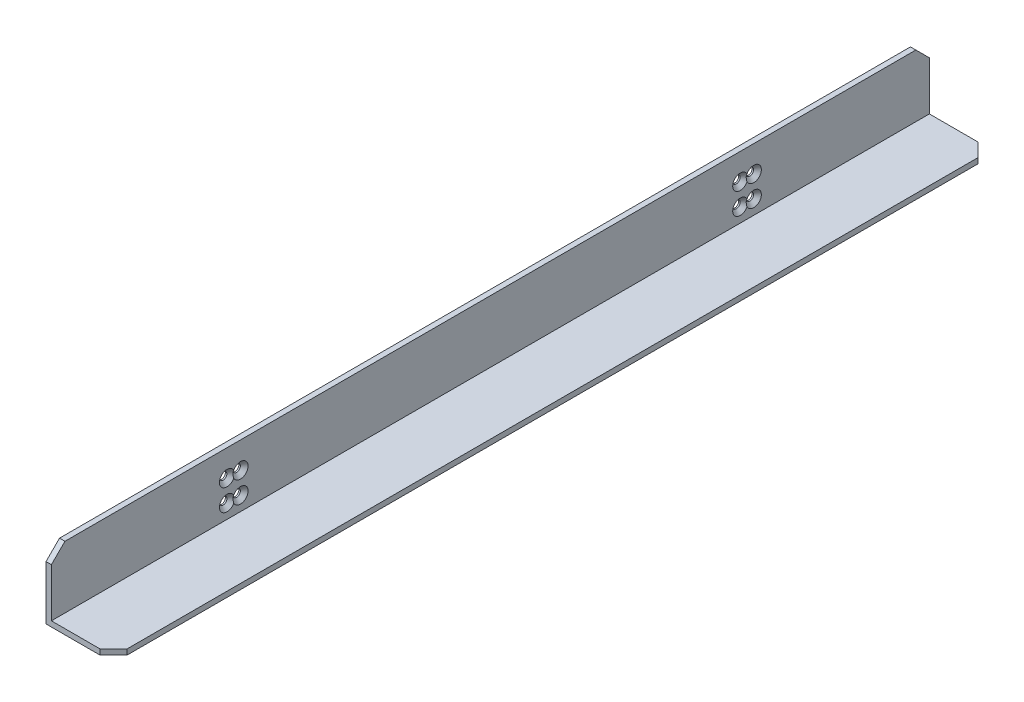
SolidWorks part; units mm, degrees
material "Q235A"
ref_plane "前视基准面" through (0, 0, 0) normal (0, 0, 1) x (1, 0, 0)
ref_plane "上视基准面" through (0, 0, 0) normal (0, 1, 0) x (1, 0, 0)
ref_plane "右视基准面" through (0, 0, 0) normal (1, 0, 0) x (0, 0, -1)
sketch "草图1" plane through (0, 0, 0) normal (0, 0, 1) x (1, 0, 0)
  line L0 (0, 0) -> (50, 0)
  line L1 (50, 0) -> (50, 4)
  line L2 (50, 4) -> (4, 4)
  line L3 (4, 4) -> (4, 50)
  line L4 (4, 50) -> (0, 50)
  line L5 (0, 50) -> (0, 0)
  dimension "D1" = 50
  dimension "D2" = 4
extrude "凸台-拉伸1" add sketch "草图1" along normal mid plane 650
chamfer "倒角1" distance 10 angle 45 4 edges at (50, 2, -325) (2, 50, -325) (50, 2, 325) (2, 50, 325)
hole_wizard "M5 六角凹锥坑螺钉的锥形沉头孔2" positions "草图4" profile "草图5" countersink size "M5" standard "ISO" end condition through all
sketch "草图4" plane through (4, 0, 0) normal (1, 0, 0) x (0, 0, -1)
  line L0 (185, 30.5) -> (195, 30.5) construction
  line L1 (185, 14.5) -> (195, 14.5) construction
  line L2 (195, 30.5) -> (195, 14.5) construction
  point P0 (-195, 30.5)
  point P3 (185, 30.5)
  point P9 (-185, 30.5)
  point P10 (195, 30.5)
  point P16 (-195, 14.5)
  point P17 (185, 14.5)
  point P18 (-185, 14.5)
  point P19 (195, 14.5)
  dimension "D2" = 10
  dimension "D4" = 16
  dimension "D1" = 2
  dimension "D3" = 2
sketch "草图5" plane through (4, 30.5, 195) normal (0, 1, 0) x (0, 0, -1)
  line L0 (0, 0) -> (0, 4)
  line L1 (0, 4) -> (2.75, 4)
  line L2 (2.75, 4) -> (2.75, 2.85)
  line L3 (2.75, 2.85) -> (5.6, 0)
  line L5 (5.6, 0) -> (0, 0)
  line L6 (-2.75, 2.85) -> (-5.6, 0) construction
  line L11 (0, -6.35) -> (0, 107.95) construction
  dimension "通孔孔直径" = 5.5
  dimension "通孔孔深度" = 4
  dimension "近端锥形沉头孔直径" = 11.2
  dimension "近端锥形沉头孔角度" = 90
